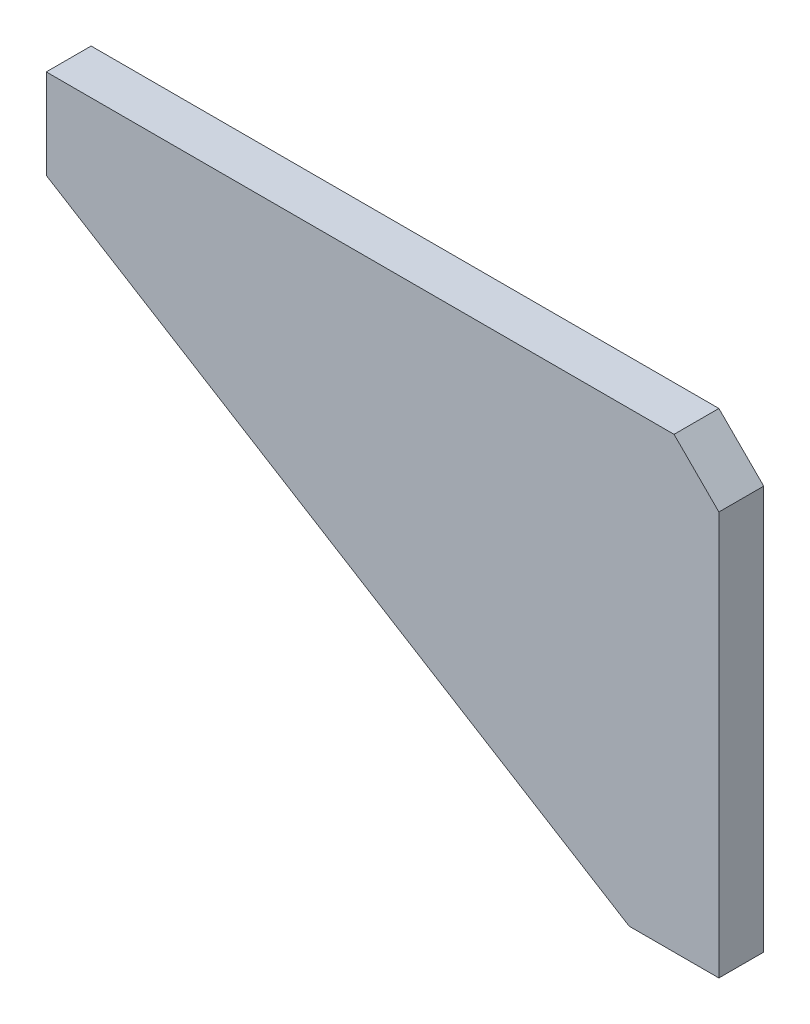
SolidWorks part; units mm, degrees
material "普通碳钢"
ref_plane "Front Plane" through (0, 0, 0) normal (0, 0, 1) x (1, 0, 0)
ref_plane "Top Plane" through (0, 0, 0) normal (0, 1, 0) x (1, 0, 0)
ref_plane "Right Plane" through (0, 0, 0) normal (1, 0, 0) x (0, 0, -1)
sketch "Sketch1" plane through (0, 0, 0) normal (0, 0, 1) x (1, 0, 0)
  line L0 (0, 0) -> (-150, 0)
  line L2 (-150, 0) -> (-150, -20)
  line L3 (-150, -20) -> (-20, -100)
  line L4 (-20, -100) -> (0, -100)
  line L6 (0, -100) -> (0, 0)
  dimension "D1" = 150
  dimension "D2" = 100
  dimension "D3" = 20
  dimension "D4" = 20
extrude "Boss-Extrude1" add sketch "Sketch1" against normal blind 10
chamfer "Chamfer1" distance 10 angle 45 1 edges at (0, 0, -5)
